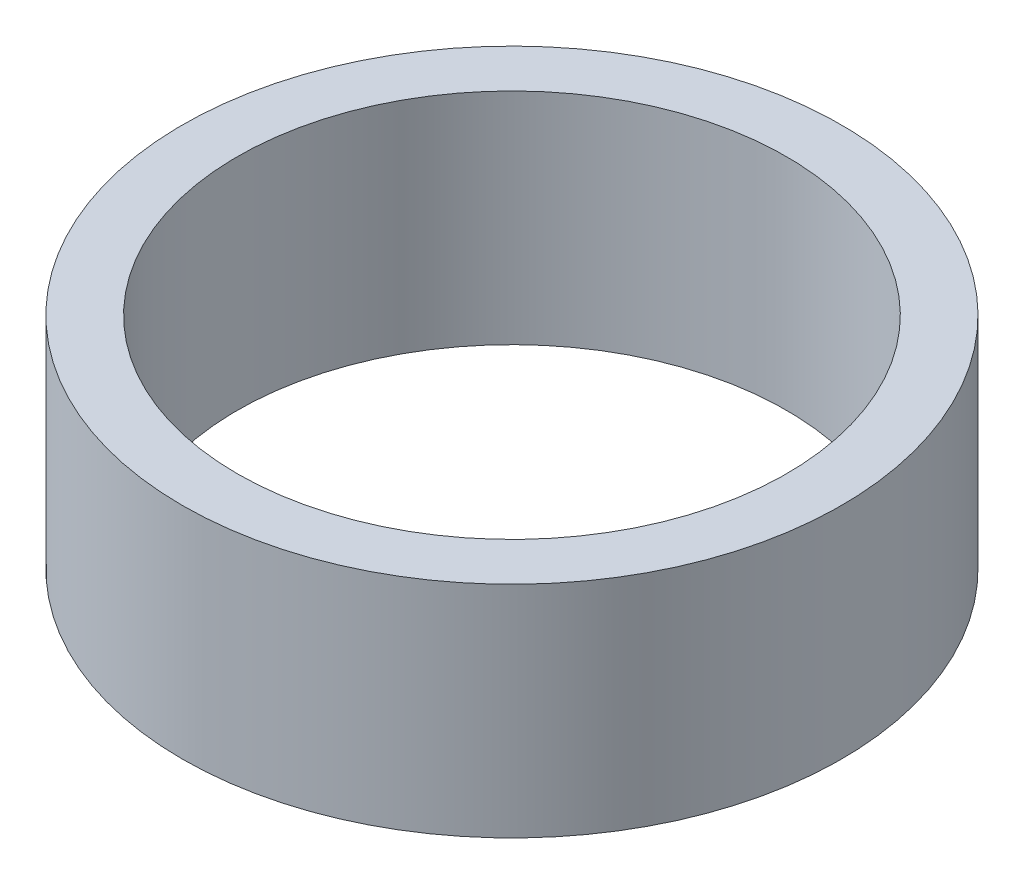
from build123d import *

# Parameters (mm, degrees)
SKETCH1_R           = 3
SKETCH1_R_2         = 2.5
BOSS_EXTRUDE1_DEPTH = 2


with BuildPart() as part:
    # Sketch1 → Boss-Extrude1 (new body)
    with BuildSketch(Plane(origin=(0, 0, 0), x_dir=(1, 0, 0), z_dir=(0, 1, 0))):
        with Locations(Location((0, 0, 0), (0, 0, 270))):
            Circle(SKETCH1_R)
        with Locations(Location((0, 0, 0), (0, 0, 270))):
            Circle(SKETCH1_R_2, mode=Mode.SUBTRACT)
    extrude(amount=BOSS_EXTRUDE1_DEPTH)


solid = part.part
